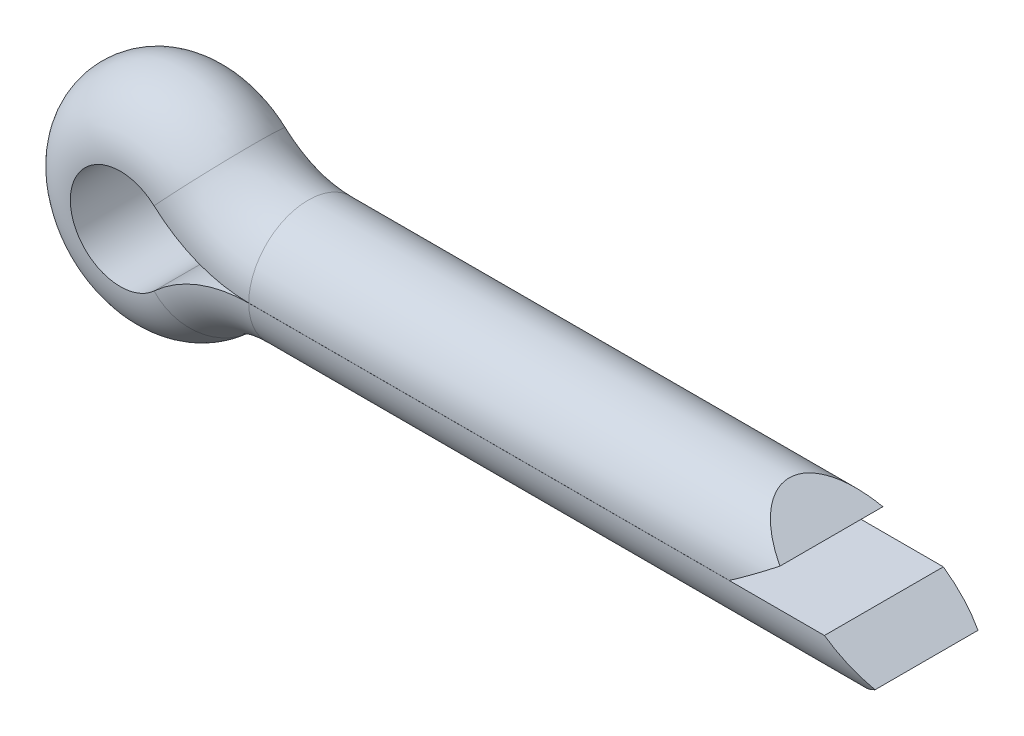
SolidWorks part; units mm, degrees
material "Q215"
ref_plane "Front" through (0, 0, 0) normal (0, 0, 1) x (1, 0, 0)
ref_plane "Top" through (0, 0, 0) normal (0, 1, 0) x (1, 0, 0)
ref_plane "Right" through (0, 0, 0) normal (1, 0, 0) x (0, 0, -1)
sketch "Sketch2" plane through (0, 0, 0) normal (0, 0, 1) x (1, 0, 0)
  line L0 (22, 2.5) -> (0, 2.5)
  line L1 (0, -2.5) -> (26, -2.5)
  line L2 (0, 0) -> (49.7718, 0) construction
  line L3 (0, 0) -> (0, 16.5256) construction
  line L4 (-10, 0) -> (-10, 14.2137) construction
  arc A0 (0, 2.5) -> (-2.2922, 3.3914) centre (0, 5.8929) cw
  arc A1 (-2.2922, 3.3914) -> (-2.2922, -3.3914) centre (-5.4, 0) ccw
  arc A2 (-2.2922, -3.3914) -> (0, -2.5) centre (0, -5.8929) cw
ref_plane "SectionPlane" through (22, 0, 0) normal (1, 0, 0) x (0, 0, -1)
sketch "Sketch1" plane through (22, 0, 0) normal (1, 0, 0) x (0, 0, -1)
  line L1 (-2.5, 0.002) -> (2.5, 0.002)
  arc A0 (2.5, 0.002) -> (-2.5, 0.002) centre (0, 0) ccw
sweep "Body" add profiles "Sketch1" path "Sketch2"
sketch "Sketch3" plane through (0, 0, 0) normal (0, 0, 1) x (1, 0, 0)
  line L0 (0, 0) -> (0, 16.2682) construction
  line L1 (0, 0) -> (75.9079, 0) construction
  line L2 (0, 0) -> (26, 0) construction
  line L3 (22, 1.251) -> (20.2105, 2.51)
  line L4 (22, 0.002) -> (22, 2.5) construction
  line L6 (22, 1.251) -> (20.2049, 0)
  line L7 (26, -1.251) -> (24.2049, 0)
  line L8 (26, -2.5) -> (26, -0.002) construction
  line L9 (26, -1.251) -> (24.2105, -2.51)
  line L10 (24.2049, 0) -> (20.2049, 0)
  line L11 (20.2105, 2.51) -> (26.01, 2.51)
  line L12 (26.01, 2.51) -> (26.01, -2.51)
  line L13 (26.01, -2.51) -> (24.2105, -2.51)
  line L14 (22, 2.5) -> (0, 2.5) construction
  dimension "D1" = 0.01
  dimension "D2" = 0.01
  dimension "D3" = 70
  dimension "D4" = 70
extrude "ConeCut" cut sketch "Sketch3" against normal through all and the other way through all
equation "' \"Diameter@Sketch2\" = 9.5"
equation "' \"Diameter@草图2\" = 9.5"
equation "' \"c@Sketch2\" = 19"
equation "' \"c@草图2\" = 19"
equation "' \"b@Sketch2\" = 20"
equation "' \"b@草图2\" = 20"
equation "' \"a@Sketch2\" = 6.3"
equation "' \"a@草图2\" = 6.3"
equation "' \"l@Sketch2\" = 45"
equation "' \"l@草图2\" = 45"
equation "' \"Diameter@Sketch2\" = 1"
equation "' \"Diameter@草图2\" = 1"
equation "' \"c@Sketch2\" = 2"
equation "' \"c@草图2\" = 2"
equation "' \"b@Sketch2\" = 3"
equation "' \"b@草图2\" = 3"
equation "' \"a@Sketch2\" = 2.5"
equation "' \"a@草图2\" = 2.5"
equation "' \"l@Sketch2\" = 8"
equation "' \"l@草图2\" = 8"
equation "' \"Diameter@Sketch2\" = 0.5"
equation "' \"Diameter@草图2\" = 0.5"
equation "' \"c@Sketch2\" = 1"
equation "' \"c@草图2\" = 1"
equation "' \"b@Sketch2\" = 2"
equation "' \"b@草图2\" = 2"
equation "' \"a@Sketch2\" = 1.6"
equation "' \"a@草图2\" = 1.6"
equation "' \"l@Sketch2\" = 4"
equation "' \"l@草图2\" = 4"
equation "\"Diameter@Sketch1\" = \"Diameter@Sketch2\""
equation "\"Length@SectionPlane\" = \"l@Sketch2\""
